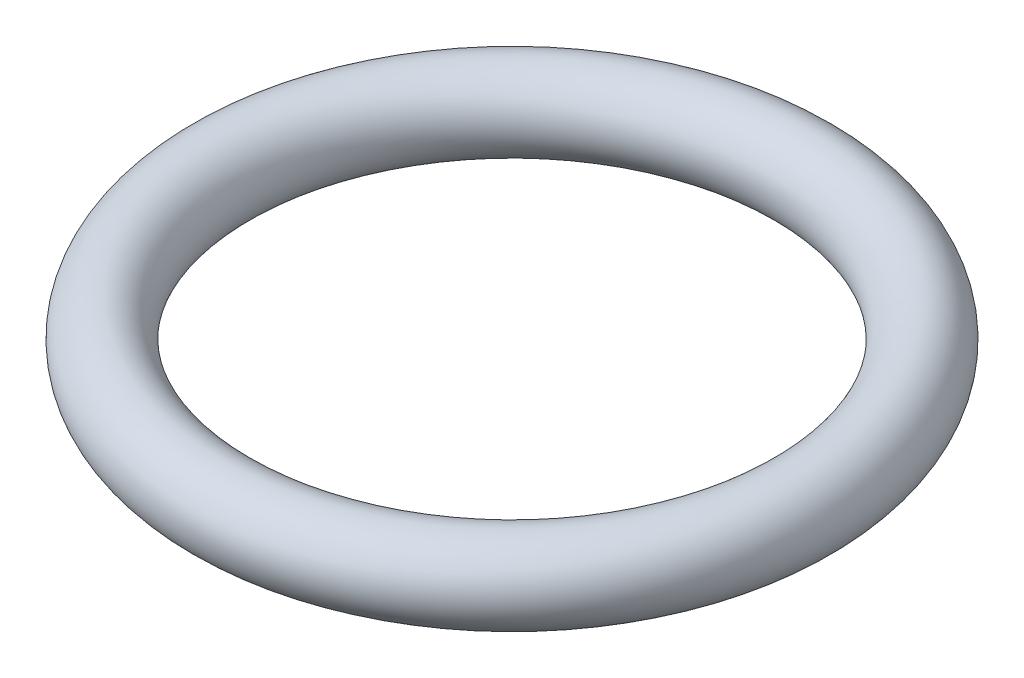
from build123d import *

# Parameters (mm, degrees)
SKETCH1_R = 15


with BuildPart() as part:
    # Sketch1 → Revolve1 (revolve)
    with BuildSketch(Plane.XY, mode=Mode.PRIVATE) as revolve1_sk:
        with Locations((110, 0)):
            Circle(SKETCH1_R)
    revolve(revolve1_sk.sketch.rotate(Axis((0, 0, 0), (0, 1, 0)), 90), axis=Axis((0, 0, 0), (0, 1, 0)))


solid = part.part
